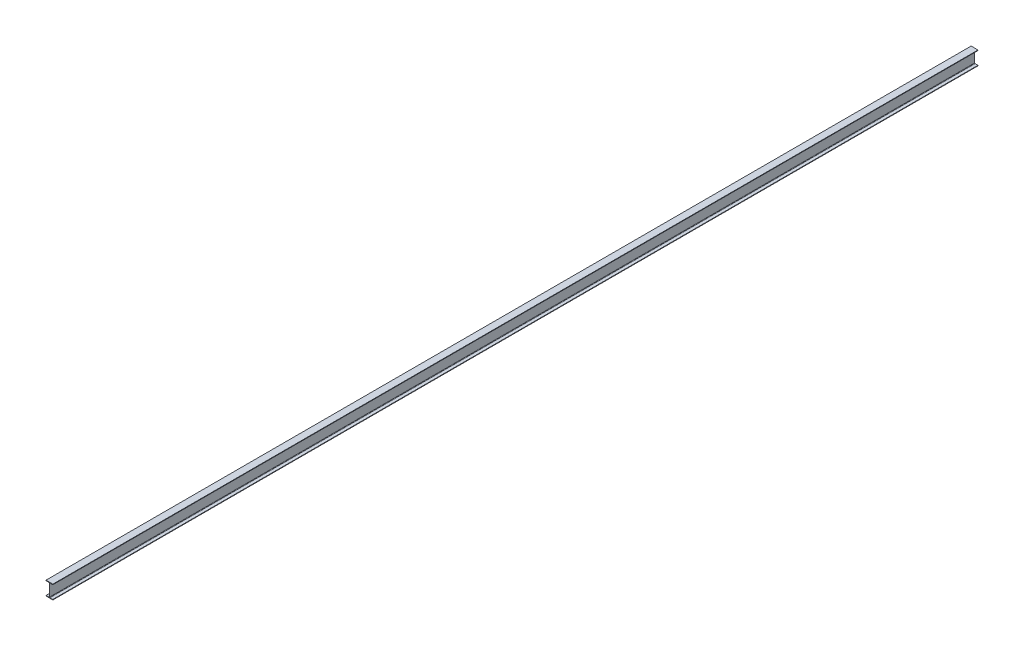
SolidWorks part; units mm, degrees
ref_plane "Front Plane" through (0, 0, 0) normal (0, 0, 1) x (1, 0, 0)
ref_plane "Top Plane" through (0, 0, 0) normal (0, 1, 0) x (1, 0, 0)
ref_plane "Right Plane" through (0, 0, 0) normal (1, 0, 0) x (0, 0, -1)
other "Configuration Table"
sketch "Sketch1" plane through (0, 0, 0) normal (0, 0, 1) x (1, 0, 0)
  line L0 (0, 0) -> (0, 250) construction
  line L1 (62.5, 0) -> (-62.5, 0)
  line L2 (-62.5, 0) -> (-62.5, 9)
  line L3 (-62.5, 9) -> (-11, 9)
  line L4 (3, 17) -> (3, 233)
  line L6 (-62.5, 241) -> (-62.5, 250)
  line L7 (-62.5, 250) -> (62.5, 250)
  line L8 (-3, 17) -> (-3, 233)
  line L9 (62.5, 241) -> (62.5, 250)
  line L10 (11, 241) -> (62.5, 241)
  line L11 (62.5, 9) -> (11, 9)
  line L12 (62.5, 0) -> (62.5, 9)
  line L13 (-11, 241) -> (-62.5, 241)
  arc A0 (11, 9) -> (3, 17) centre (11, 17) cw
  arc A1 (-3, 17) -> (-11, 9) centre (-11, 17) cw
  arc A2 (3, 233) -> (11, 241) centre (11, 233) cw
  arc A3 (-3, 233) -> (-11, 241) centre (-11, 233) ccw
  point P18 (3, 9)
  point P21 (-3, 9)
  point P24 (3, 241)
  point P27 (-3, 241)
  dimension "D6" = 8
  dimension "D1" = 250
  dimension "D2" = 125
  dimension "D3" = 6
  dimension "D4" = 9
  dimension "D5" = 9
extrude "Boss-Extrude1" add sketch "Sketch1" along normal blind 16840
